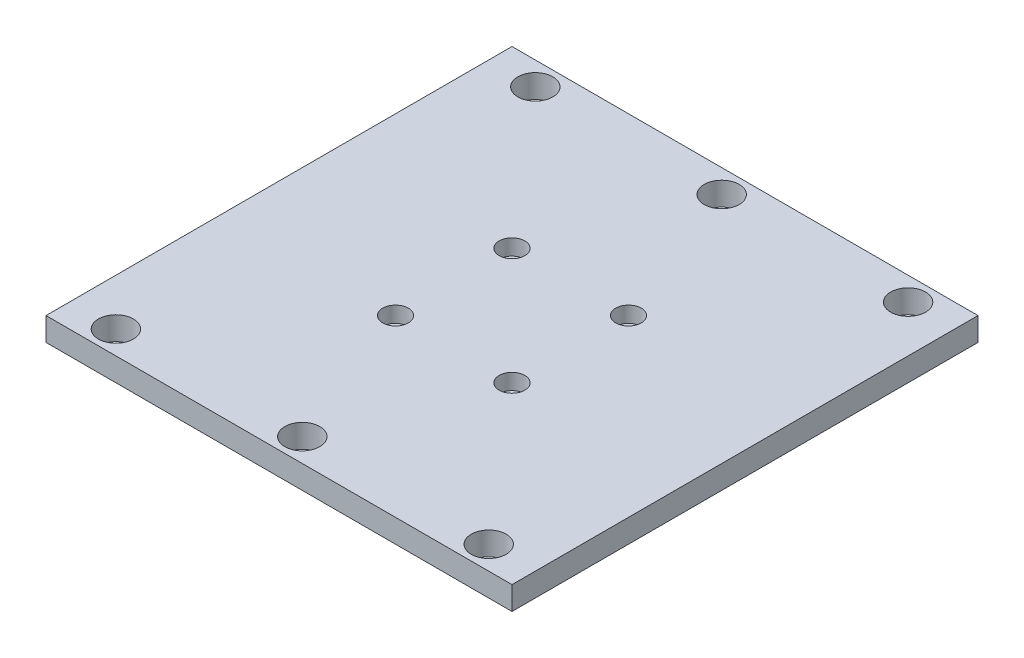
SolidWorks part; units mm, degrees
ref_plane "Front Plane" through (0, 0, 0) normal (0, 0, 1) x (1, 0, 0)
ref_plane "Top Plane" through (0, 0, 0) normal (0, 1, 0) x (1, 0, 0)
ref_plane "Right Plane" through (0, 0, 0) normal (1, 0, 0) x (0, 0, -1)
sketch "Sketch1" plane through (0, 0, 0) normal (0, 1, 0) x (1, 0, 0)
  line L1 (-100, 100) -> (100, 100)
  line L2 (-100, 100) -> (-100, -100)
  line L3 (-100, -100) -> (100, -100)
  line L4 (100, 100) -> (100, -100)
  line L5 (-100, 100) -> (100, -100) construction
  line L6 (-100, -100) -> (100, 100) construction
  point P0 (0, 0)
  dimension "D1" = 200
  dimension "D2" = 200
extrude "Boss-Extrude1" add sketch "Sketch1" along normal mid plane 10
sketch "Sketch2" plane through (0, 5, 0) normal (0, 1, 0) x (1, 0, 0)
  line L0 (0, 90) -> (0, -90) construction
  line L1 (80, 90) -> (-80, 90) construction
  line L2 (80, 90) -> (80, -90) construction
  line L3 (80, -90) -> (-80, -90) construction
  line L4 (-80, 90) -> (-80, -90) construction
  line L5 (80, 90) -> (-80, -90) construction
  line L6 (80, -90) -> (-80, 90) construction
  circle A0 centre (80, 90) radius 7.5
  point P0 (0, 0)
  dimension "D3" = 15
  dimension "D1" = 180
  dimension "D2" = 160
extrude "Cut-Extrude1" cut sketch "Sketch2" against normal blind 10
pattern_linear "LPattern1" count 2 spacing 180 along (0, 0, 1) count 3 spacing 80 along (-1, 0, 0) of "Cut-Extrude1"
sketch "Sketch3" plane through (0, 5, 0) normal (0, 1, 0) x (1, 0, 0)
  line L1 (25, 25) -> (-25, 25) construction
  line L2 (25, 25) -> (25, -25) construction
  line L3 (25, -25) -> (-25, -25) construction
  line L4 (-25, 25) -> (-25, -25) construction
  line L5 (25, 25) -> (-25, -25) construction
  line L6 (25, -25) -> (-25, 25) construction
  point P0 (0, 0)
  dimension "D1" = 50
  dimension "D2" = 50
hole_wizard "Hole Size (based on socket head cap screw type)1" positions "Sketch4" profile "Sketch5" counterbore size "M6" standard "GB" end condition up to next
sketch "Sketch4" plane through (0, 5, 0) normal (0, 1, 0) x (1, 0, 0)
  point P0 (25, 25)
  point P3 (25, -25)
  point P6 (-25, 25)
  point P9 (-25, -25)
sketch "Sketch5" plane through (25, 5, -25) normal (1, 0, 0) x (0, 0, 1)
  line L0 (0, 0) -> (0, 10)
  line L1 (0, 10) -> (3.3, 10)
  line L3 (3.3, 10) -> (3.3, 6.8)
  line L4 (3.3, 6.8) -> (5.5, 6.8)
  line L5 (5.5, 6.8) -> (5.5, 0)
  line L7 (5.5, 0) -> (0, 0)
  line L11 (0, -6.35) -> (0, 107.95) construction
  dimension "通孔孔直径" = 6.6
  dimension "通孔孔深度" = 10
  dimension "柱形沉头孔直径" = 11
  dimension "柱形沉头孔深度" = 6.8
